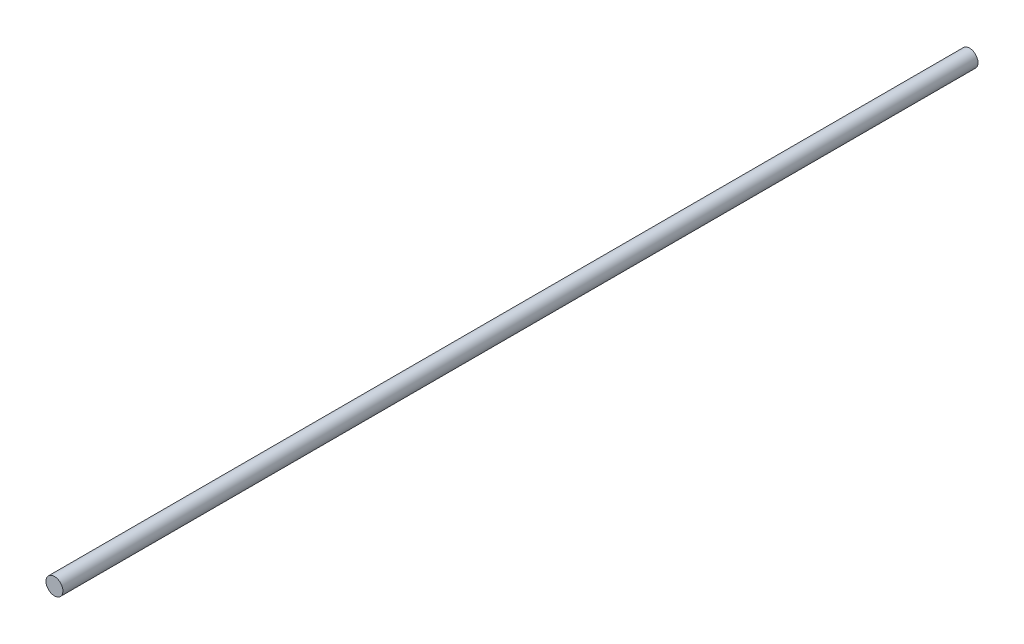
from build123d import *

# Parameters (mm, degrees)
SKETCH_1_R      = 12.5
EXTRUDE_1_DEPTH = 1352


with BuildPart() as part:
    # 草图1 → 凸台-拉伸1 (new body)
    with BuildSketch(Plane.XY):
        Circle(SKETCH_1_R)
    extrude(amount=EXTRUDE_1_DEPTH)


solid = part.part
